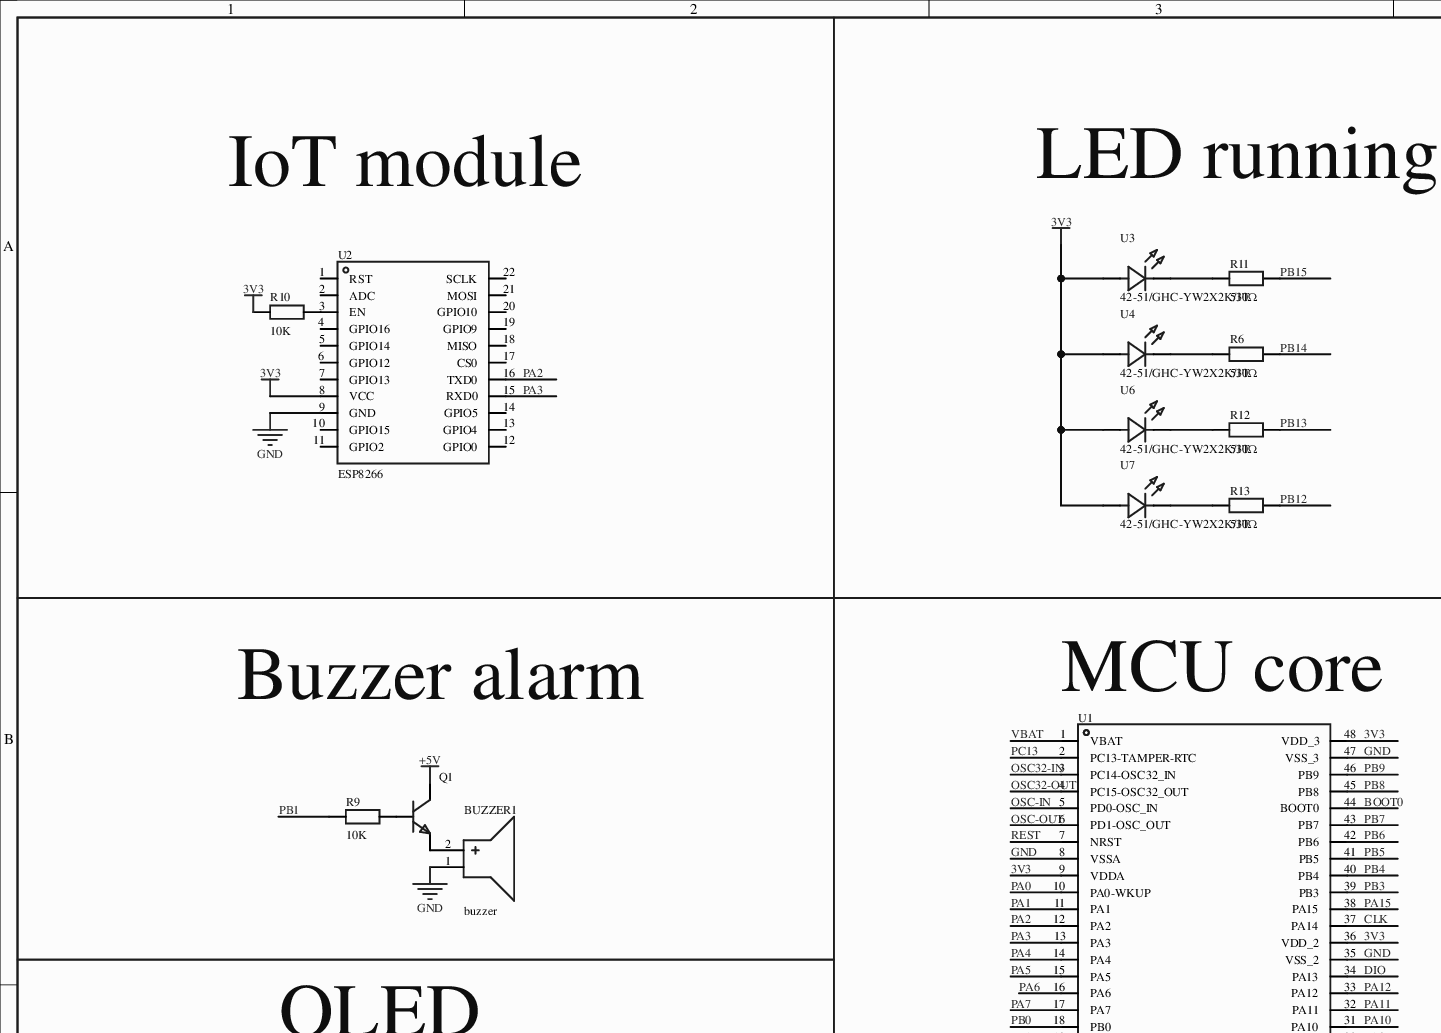
[diagram p0: MISC61952-3.schdoc, top left]
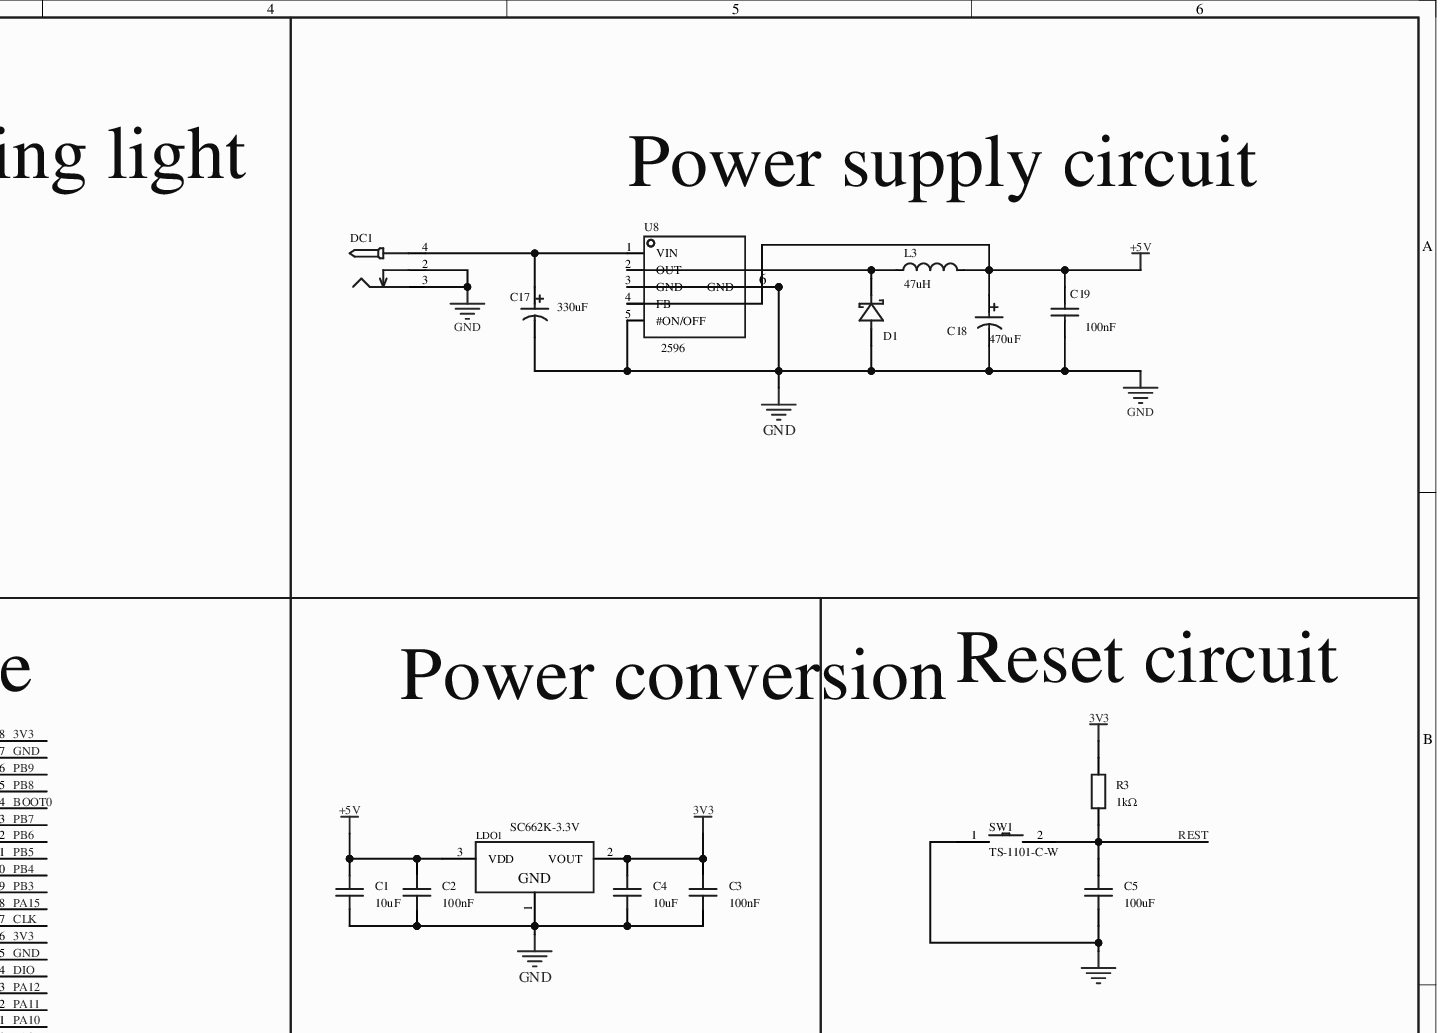
[diagram p1: MISC61952-3.schdoc, top right]
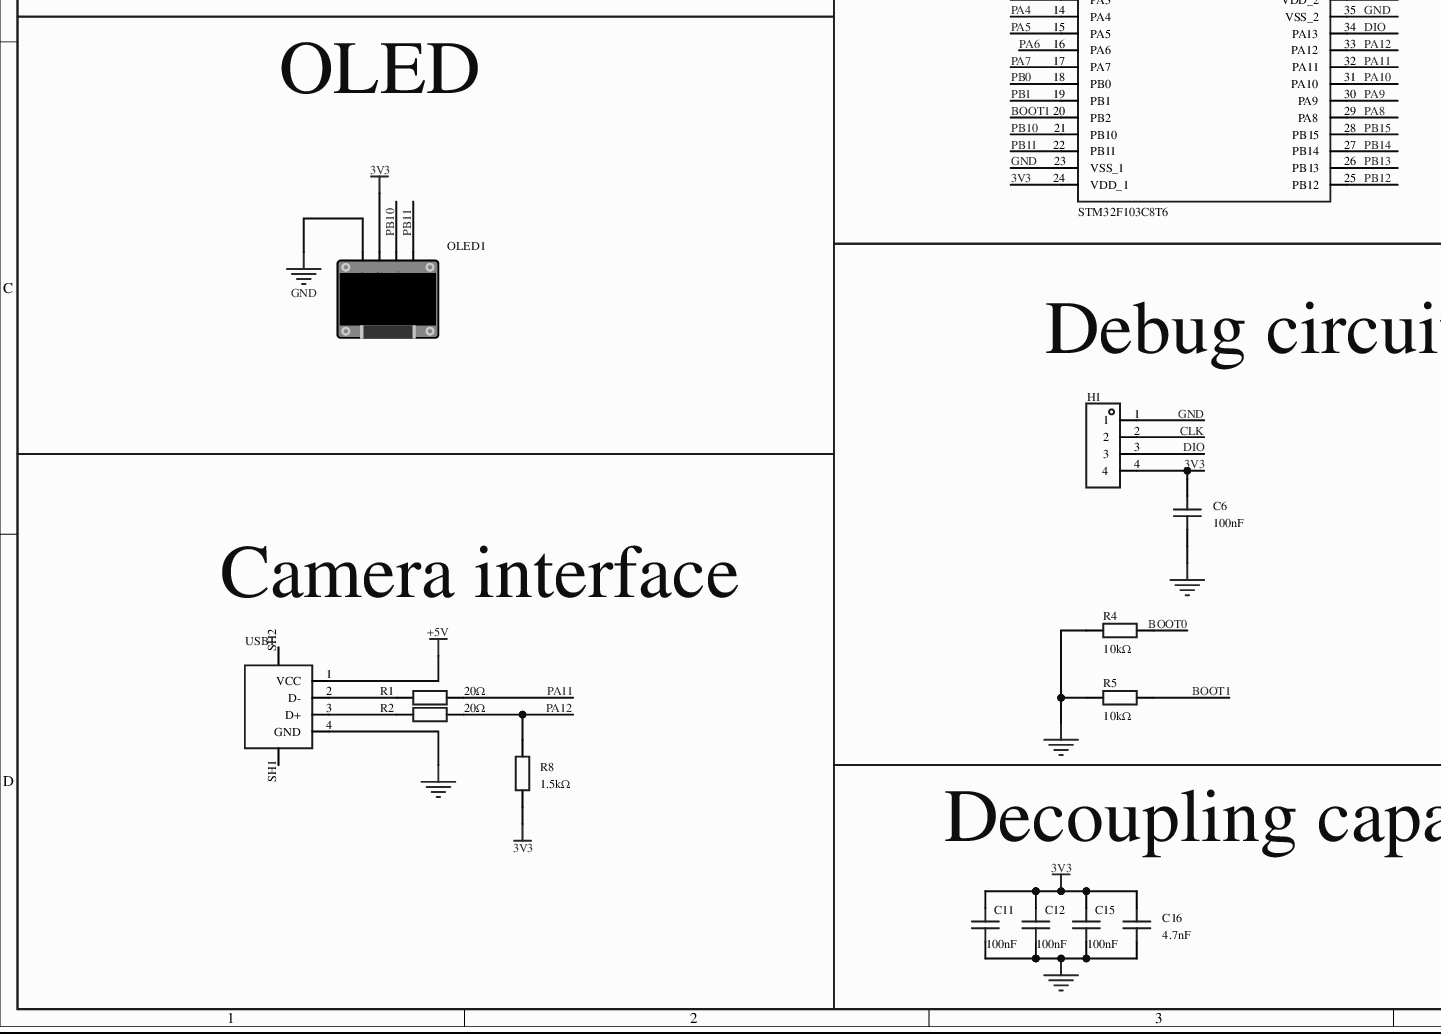
[diagram p2: MISC61952-3.schdoc, bottom left]
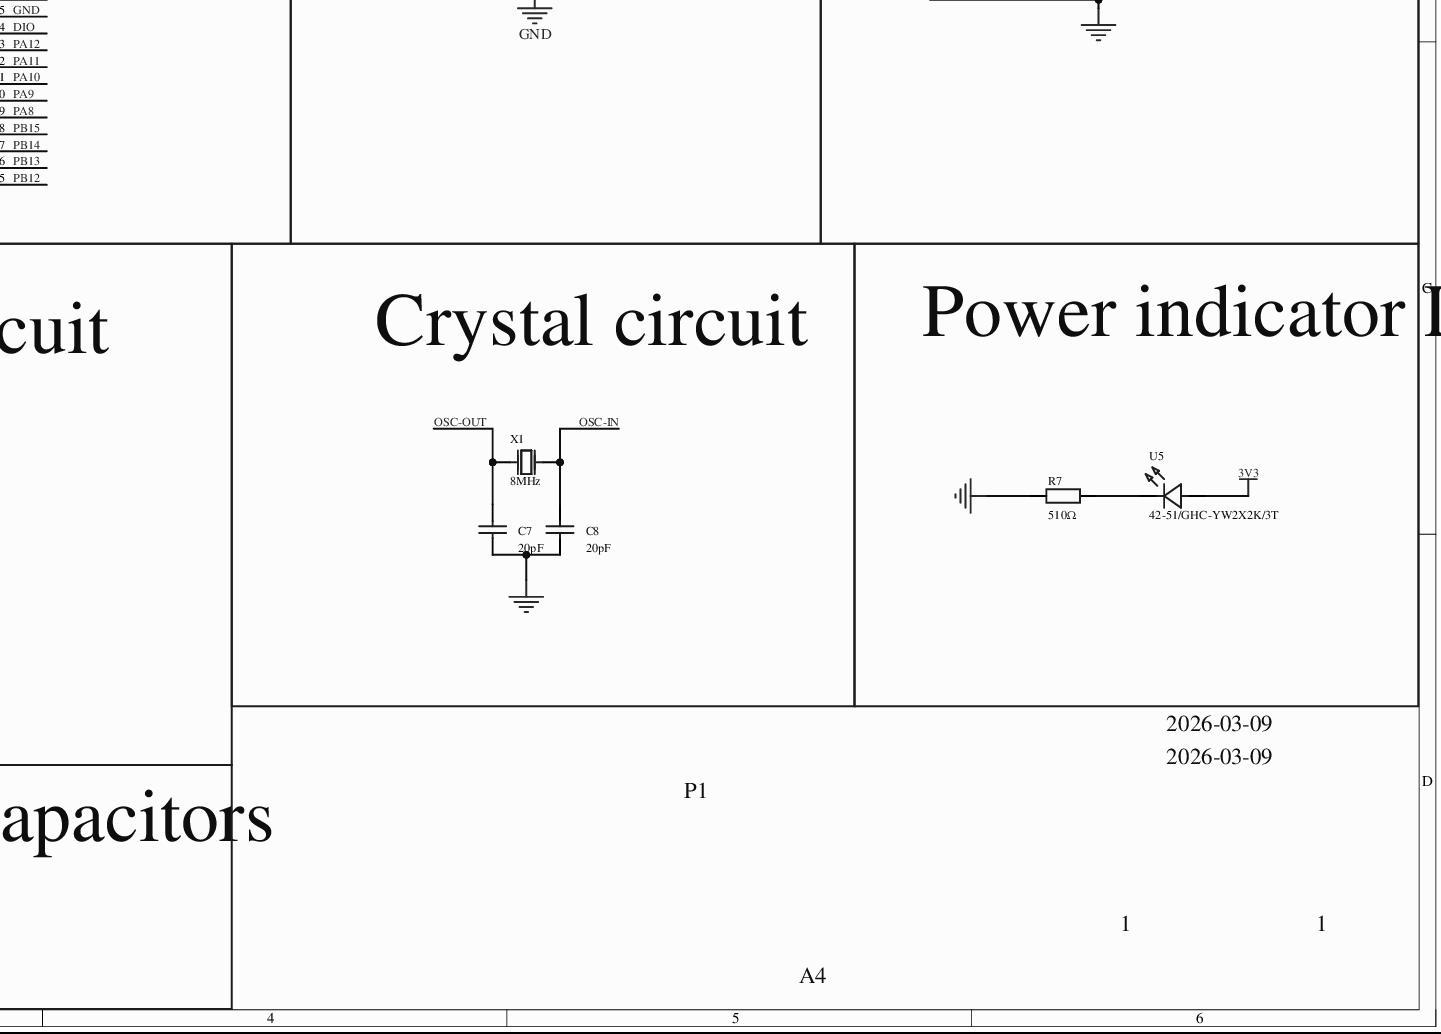
[diagram p3: MISC61952-3.schdoc, bottom right]
# Altium project MISC61952-2.PrjPcb
1 sheet, 47 parts. Net scope: global (net labels, ports and power ports of the same name join across sheets).
Board file: MISC61952.pcbdoc

## Sheet MISC61952-3.schdoc
size 420 x 297 mm; Version: V1.0; @Project Name: MISC61952; @Page Count: 1; @Update Date: 2026-03-09; @Create Date: 2026-03-09; @Schematic Name: MISC61952; @Page No: 1; @Board Name: MISC61952; @Create Time: 07:18:17; @Update Time: 19:34:13

### Parts
BUZZER1  buzzer  [BUZ-TH_BD12.0-P6.00-D0.9-RD]
C1  10uF  [C0603]
C2  100nF  [C0603]
C3  100nF  [C0603]
C4  10uF  [C0603]
C5  100uF  [C1206]
C6  100nF  [C0603]
C7  20pF  [C0603]
C8  20pF  [C0603]
C11  100nF  [C0603]
C12  100nF  [C0603]
C15  100nF  [C0603]
C16  4.7nF  [C0603]
C17  value 330uF  [CAP-SMD_BD8.0-L8.3-W8.3-RD]
C18  value 470uF  [CAP-SMD_BD8.0-L8.3-W8.3-RD]
C19  value 100nF  [C0805]
D1  (no value)  [SMA_L4.3-W2.6-LS5.2-RD]
DC1  (no value)  [DC-2.0]
H1  (no value)  [HDR-TH_4P-P2.54-V-M]
L3  value 47uH  [IND-SMD_L7.0-W6.6]
LDO1  SC662K-3.3V  [SOT-23-3_L2.9-W1.3-P1.90-LS2.4-BR]
OLED1  (no value)  [0.96OLED_4P]
Q1  (no value)  [S8050_SOT-23]
R1  20Ω  [R0603]
R2  20Ω  [R0603]
R3  1kΩ  [R0603]
R4  10kΩ  [R0603]
R5  10kΩ  [R0603]
R6  510Ω  [R0603]
R7  510Ω  [R0603]
R8  1.5kΩ  [R0603]
R9  10K  [R0603]
R10  10K  [R0603]
R11  510Ω  [R0603]
R12  510Ω  [R0603]
R13  510Ω  [R0603]
SW1  TS-1101-C-W  [SW-SMD_L6.0-W3.3-LS8.0]
U1  STM32F103C8T6  [LQFP-48_L7.0-W7.0-P0.50-LS9.0-BL]
U2  ESP8266  [WIFIM-SMD_ESP-12F-ESP8266MOD]
U3  42-51/GHC-YW2X2K/3T  [LED-SMD_L1.6-W0.8-FD_GREEN-1]
U4  42-51/GHC-YW2X2K/3T  [LED-SMD_L1.6-W0.8-FD_GREEN-1]
U5  42-51/GHC-YW2X2K/3T  [LED-SMD_L1.6-W0.8-FD_GREEN-1]
U6  42-51/GHC-YW2X2K/3T  [LED-SMD_L1.6-W0.8-FD_GREEN-1]
U7  42-51/GHC-YW2X2K/3T  [LED-SMD_L1.6-W0.8-FD_GREEN-1]
U8  LM2596S-5.0  [TO-263-5_L10.2-W8.9-P1.70-BR]  (value not drawn)
USB1  (no value)  [USB_ Type-A]
X1  8MHz  [OSC-TH_L10.0-W4.5-P5.00]

### Blocks framed on the sheet
IoT module: R10 U2
LED running light: R6 R11-R13 U3 U4 U6 U7
Power supply circuit: C17-C19 D1 DC1 L3 U8
Buzzer alarm: BUZZER1 Q1 R9
MCU core: U1
Power conversion: C1-C4 LDO1
Reset circuit: C5 R3 SW1
OLED: OLED1
Debug circuit: C6 H1 R4 R5
Crystal circuit: C7 C8 X1
Power indicator LED: R7 U5
Camera interface: R1 R2 R8 USB1
Decoupling capacitors: C11 C12 C15 C16

### Nets
3V3: C3.2 C4.2 C6.2 C11.2 C12.2 C15.2 C16.2 H1.4 LDO1.2(VOUT) OLED1.2(VCC) R3.2 R8.1 R10.1 U1.9(VDDA) U1.24(VDD_1) U1.36(VDD_2) U1.48(VDD_3) U2.8(VCC) U3.1(A) U4.1(A) U5.1(A) U6.1(A) U7.1(A)
+5V: C1.2 C2.2 C18.1 C19.1 L3.2 LDO1.3(VDD) Q1.3 U8.4(FB) USB1.1(VCC)
GND: BUZZER1.1(-) C1.1 C2.1 C3.1 C4.1 C5.1 C6.1 C7.1 C8.1 C11.1 C12.1 C15.1 C16.1 C17.2 C18.2 C19.2 D1.2(A) DC1.2 DC1.3 H1.1 LDO1.1(GND) OLED1.1(GND) R4.1 R5.1 R7.2 SW1.1 U1.8(VSSA) U1.23(VSS_1) U1.35(VSS_2) U1.47(VSS_3) U2.9(GND) U8.3(GND) U8.5(#ON/OFF) U8.6(GND) USB1.4(GND)
BOOT0: R4.2 U1.44(BOOT0)
BOOT1: R5.2 U1.20(PB2)
CLK: H1.2 U1.37(PA14)
DIO: H1.3 U1.34(PA13)
OSC32-IN: U1.3(PC14-OSC32_IN)
OSC32-OUT: U1.4(PC15-OSC32_OUT)
OSC-IN: C8.2 U1.5(PD0-OSC_IN) X1.1(OSC1)
OSC-OUT: C7.2 U1.6(PD1-OSC_OUT) X1.2(OSC2)
PA0: U1.10(PA0-WKUP)
PA1: U1.11(PA1)
PA2: U1.12(PA2) U2.16(TXD0)
PA3: U1.13(PA3) U2.15(RXD0)
PA4: U1.14(PA4)
PA5: U1.15(PA5)
PA6: U1.16(PA6)
PA7: U1.17(PA7)
PA8: U1.29(PA8)
PA9: U1.30(PA9)
PA10: U1.31(PA10)
PA11: R1.2 U1.32(PA11)
PA12: R2.2 R8.2 U1.33(PA12)
PA15: U1.38(PA15)
PB0: U1.18(PB0)
PB1: R9.1 U1.19(PB1)
PB3: U1.39(PB3)
PB4: U1.40(PB4)
PB5: U1.41(PB5)
PB6: U1.42(PB6)
PB7: U1.43(PB7)
PB8: U1.45(PB8)
PB9: U1.46(PB9)
PB10: OLED1.3(SCL) U1.21(PB10)
PB11: OLED1.4(SDA) U1.22(PB11)
PB12: R13.2 U1.25(PB12)
PB13: R12.2 U1.26(PB13)
PB14: R6.2 U1.27(PB14)
PB15: R11.2 U1.28(PB15)
PC13: U1.2(PC13-TAMPER-RTC)
REST: C5.2 R3.1 SW1.2 U1.7(NRST)
VBAT: U1.1(VBAT)
NetBUZZER1_2: BUZZER1.2(+) Q1.2
NetC17_1: C17.1 DC1.4 U8.1(VIN)
NetD1_1: D1.1(K) L3.1 U8.2(OUT)
NetQ1_1: Q1.1 R9.2
NetR1_1: R1.1 USB1.2(D-)
NetR2_1: R2.1 USB1.3(D+)
NetR6_1: R6.1 U4.2(C)
NetR7_1: R7.1 U5.2(C)
NetR10_2: R10.2 U2.3(EN)
NetR11_1: R11.1 U3.2(C)
NetR12_1: R12.1 U6.2(C)
NetR13_1: R13.1 U7.2(C)

Not connected (* = marked no-connect by the designer): U2 1(RST) 2(ADC) 4(GPIO16) 5(GPIO14) 6(GPIO12) 7(GPIO13) 10(GPIO15) 11(GPIO2) 12(GPIO0) 13(GPIO4) 14(GPIO5) 17(CS0) 18(MISO) 19(GPIO9) 20(GPIO10) 21(MOSI) 22(SCLK); USB1 SH1 SH2

### Notes on the sheet
- 2026-03-09
- P1
- A4
- 1

### Library data of the parts
BUZZER1 = buzzer: AddInBom: yes; ModelId: af17e4151ed84fc2a628230bf23763630819f05c4eef4c71ace90d822a990e87; ModelTransform: 472.44,472.176,0,270,0,0,0,0,-196.85; Symbol: BUZZER; Device: buzzer; LCSC Part Name: buzzer; SupplierPart: C9900014030; ManufacturerPart: buzzer; Supplier Footprint: buzzer; JLCPCB Part Class: Extended Part; Supplier: LCSC; ConvertToPcb: yes; FootprintName: BUZ-TH_BD12.0-P6.00-D0.9-RD; ModelName: BUZ-TH_BD12.0-P6.00-D0.9-RD
C1 C4 = CL10A106KP8NNNC: Capacitance: 10uF; tolerance: ±10%; rated voltage: 10V; dielectric (temperature coefficient): X5R;; Manufacturer: SAMSUNG(三星); AddInBom: yes; ModelId: ac125912035d415993ca9572d50418b1; ModelName: C0603_L1.6-W0.8-H0.8; ModelTransform: 62.992,31.496,0,0,0,0,0,0,0; Device: CL10A106KP8NNNC; Symbol: CL10A106KP8NNNC; LCSC Part Name: 10uF ±10% 10V; SupplierPart: C19702; ManufacturerPart: CL10A106KP8NNNC; Supplier Footprint: 0603; JLCPCB Part Class: Basic library; Datasheet: example.com/upload/public/pdf/source/20160103/1457707703378.pdf; Supplier: LCSC; ConvertToPcb: yes; FootprintName: C0603; Value: 10uF; Tolerance: ±10%; Voltage Rated: 10V; Temperature Coefficient: X5R
C2 C3 = CC0603KRX7R9BB104: Capacitance: 100nF; tolerance: ±10%; rated voltage: 50V; dielectric (temperature coefficient): X7R;; Manufacturer: YAGEO(国巨); AddInBom: yes; ModelId: ac125912035d415993ca9572d50418b1; ModelName: C0603_L1.6-W0.8-H0.8; ModelTransform: 62.992,31.496,0,0,0,0,0,0,0; Device: CC0603KRX7R9BB104; Symbol: CC0603KRX7R9BB104; LCSC Part Name: 100nF ±10% 50V; SupplierPart: C14663; ManufacturerPart: CC0603KRX7R9BB104; Supplier Footprint: 0603; JLCPCB Part Class: Basic library; Datasheet: example.com/upload/public/pdf/source/20180910/C282072_33301C7F631E79921B82A8DAC6BCC5B3.pdf; Supplier: LCSC; ConvertToPcb: yes; FootprintName: C0603; Value: 100nF; Tolerance: ±10%; Voltage Rated: 50V; Temperature Coefficient: X7R
C5 = HGC1206R5107M100NSPJ: Capacitance: 100uF; tolerance: ±20%; rated voltage: 10V; dielectric (temperature coefficient): X5R;; Manufacturer: Chinocera(华瓷); AddInBom: yes; ModelId: e4be705b945545a48e666415e3682bd8; ModelName: C1206_L3.2-W1.6-H1.3; ModelTransform: 125.984,62.992,0,0,0,0,0,0,0; Symbol: HGC1206R5107M100NSPJ; Device: HGC1206R5107M100NSPJ; LCSC Part Name: 100uF ±20% 10V; SupplierPart: C7432784; ManufacturerPart: HGC1206R5107M100NSPJ; Supplier Footprint: 1206; JLCPCB Part Class: Extended library; Datasheet: example.com/upload/public/pdf/source/20240320/FAC3FEC40A78BC5CCCE96C232A94D860.pdf; Supplier: LCSC; ConvertToPcb: yes; FootprintName: C1206; Value: 100uF; Tolerance: ±20%; Voltage Rated: 10V; Temperature Coefficient: X5R
C6 C11 C12 C15 = CGA0603X7R104K500JT: Capacitance: 100nF; tolerance: ±10%; rated voltage: 50V; dielectric (temperature coefficient): X7R;; Manufacturer: HRE(芯声); AddInBom: yes; ModelId: ac125912035d415993ca9572d50418b1; ModelName: C0603_L1.6-W0.8-H0.8; ModelTransform: 62.992,31.496,0,0,0,0,0,0,0; Symbol: CGA0603X7R104K500JT; Device: CGA0603X7R104K500JT; LCSC Part Name: 100nF ±10% 50V; SupplierPart: C6119867; ManufacturerPart: CGA0603X7R104K500JT; Supplier Footprint: 0603; JLCPCB Part Class: Extended library; Supplier: LCSC; ConvertToPcb: yes; FootprintName: C0603; Value: 100nF; Tolerance: ±10%; Voltage Rated: 50V; Temperature Coefficient: X7R
C7 C8 = CL10C200JB8NNNC: Capacitance: 20pF; tolerance: ±5%; rated voltage: 50V; dielectric (temperature coefficient): C0G;; Manufacturer: SAMSUNG(三星); AddInBom: yes; ModelId: ac125912035d415993ca9572d50418b1; ModelName: C0603_L1.6-W0.8-H0.8; ModelTransform: 62.992,31.496,0,0,0,0,0,0,0; Symbol: CL10C200JB8NNNC; Device: CL10C200JB8NNNC; LCSC Part Name: 20pF ±5% 50V; SupplierPart: C1648; ManufacturerPart: CL10C200JB8NNNC; Supplier Footprint: 0603; JLCPCB Part Class: Basic library; Datasheet: example.com/upload/public/pdf/source/20160218/1457707763339.pdf; Supplier: LCSC; ConvertToPcb: yes; FootprintName: C0603; Value: 20pF; Tolerance: ±5%; Voltage Rated: 50V; Temperature Coefficient: C0G
C16 = CGA0603X7R472K500JT: Capacitance: 4.7nF; tolerance: ±10%; rated voltage: 50V; dielectric (temperature coefficient): X7R;; Manufacturer: HRE(芯声); AddInBom: yes; ModelId: ac125912035d415993ca9572d50418b1; ModelName: C0603_L1.6-W0.8-H0.8; ModelTransform: 62.992,31.496,0,0,0,0,0,0,0; Symbol: CGA0603X7R472K500JT; Device: CGA0603X7R472K500JT; LCSC Part Name: 4.7nF ±10% 50V; SupplierPart: C7503499; ManufacturerPart: CGA0603X7R472K500JT; Supplier Footprint: 0603; JLCPCB Part Class: Extended library; Supplier: LCSC; ConvertToPcb: yes; FootprintName: C0603; Value: 4.7nF; Tolerance: ±10%; Voltage Rated: 50V; Temperature Coefficient: X7R
C17 C18 = CS1V221M-CRF10　: Capacitance: 220uF; tolerance: ±20%; rated voltage: 35V; can diameter: 8mm; can length: 10.5mm; ripple current: -; ESR: -; operating life: 2000hrs@105; operating temperature: -40~+105;; Manufacturer: ST(先科); Rated Voltage: 25V; 3D Model: b102f1362be24624a1b1334fec8dc7f4; 3D Model Transform: 354.33,326.81037,0,0,0,0,0,0,0; AddInBom: yes; Symbol: CS1V221M-CRF10; Device: CS1V221M-CRF10; Lifetime @ Temp: 2000hrs@105; Operating Temperature: -40~+105; Manufacturer Part: CS1V221M-CRF10; Supplier Footprint: SMD,8x10.5mm; JLCPCB Part Class: Extended Part; Datasheet: example.com/upload/public/pdf/source/20170325/1490427945143.pdf; Supplier: LCSC; Tolerance: ±20%; φD: 8mm; L: 10.5mm; Ripple Current: -; Equivalent Series Resistance(ESR): -; ConvertToPcb: yes; FootprintName: CAP-SMD_BD8.0-L8.3-W8.3-RD; ModelName: CAP-SMD_BD8.0-L8.3-W8.3-RD
  C17: Supplier Part: C97814
C19 = CL21B104KBCNNNC: Capacitance: 100nF; tolerance: ±10%; rated voltage: 50V; temperature coefficient: X7R;; Manufacturer: SAMSUNG(三星); 3D Model: 1ba041120af144c991958decab20d241; 3D Model Transform: 78.74,51.181,0,0,0,0,0,0.0005,0; AddInBom: yes; ModelName: C0805_L2.0-W1.3-H1.3; Symbol: CL21B104KBCNNNC; Device: CL21B104KBCNNNC; LCSC Part Name: 100nF ±10% 50V; Supplier Part: C1711; Manufacturer Part: CL21B104KBCNNNC; Supplier Footprint: 0805; JLCPCB Part Class: Extended Part; Datasheet: example.com/upload/public/pdf/source/20160103/1457707693305.pdf; Supplier: LCSC; Tolerance: ±10%; Voltage Rated: 50V; Temperature Coefficient: X7R; ConvertToPcb: yes; FootprintName: C0805
D1 = SS34_3: Manufacturer: TDD(台冠电子); Manufacturer Part: SS34; Symbol: SS34_C3032484; 3D Model: 7ed2c9d0a4a74bbdbba07ab4052caf5b; 3D Model Transform: 185.039,102.362,0,0,0,0,0,0,0; AddInBom: yes; Device: SS34_3; LCSC Part Name: SS34; Supplier Part: C3032484; Supplier Footprint: SMA; JLCPCB Part Class: Extended Part; Datasheet: example.com/upload/public/pdf/source/20220622/9D70D0693761B542BF6F533590093AA5.pdf; Supplier: LCSC; ConvertToPcb: yes; FootprintName: SMA_L4.3-W2.6-LS5.2-RD; ModelName: SMA_L4.3-W2.6-LS5.2-RD
DC1 = DC-005_2.0: Symbol: DC power jack; ConvertToPcb: yes; ModelId: f5f20b8a2308479b936ba3c2698865bb0819f05c4eef4c71ace90d822a990e87; ModelName: DC-IN-TH_DC-5520-1; ModelTransform: 372.05,551.18,582.68,90,0,0,137.8,0,-149.61; Device: DC-005_2.0; AddInBom: yes; Supplier Footprint: 插件; FootprintName: DC-2.0
H1 = HDR-M_2.54_1x4P: Symbol: PZ254V-11-04P; ConvertToPcb: yes; ModelId: 112f4d05e8d64e99ab9a333894bea4f90819f05c4eef4c71ace90d822a990e87; ModelName: HDR-TH_4P-P2.54-M-LI-1X4P; ModelTransform: 399.999,104.7242,0,0,0,0,0,0,-118.11; Device: HDR-M_2.54_1x4P; AddInBom: yes; SupplierPart: C492403; Supplier Footprint: 插件; FootprintName: HDR-TH_4P-P2.54-V-M
L3 = CMLO0630H330MTT: Inductance: 33uH; tolerance: ±20%; DC resistance (DCR): 270mΩ;; Manufacturer: Cybermax(思博科技); 3D Model: 6860c29aec394a38a0f014af7f722a42; 3D Model Transform: 275.6,259.8,0,0,0,0,0,0,0; AddInBom: yes; ModelName: IND-SMD_L7.0-W6.6-H3.0; Symbol: CMLO0630H330MTT; Device: CMLO0630H330MTT; LCSC Part Name: 33uH ±20% 270mΩ; Manufacturer Part: CMLO0630H330MTT; Supplier Footprint: SMD; JLCPCB Part Class: Extended Part; Datasheet: example.com/upload/public/pdf/source/20201124/C961478_55C23F293F63DC1D2CF3D7AB16D0E182.pdf; Supplier: LCSC; Tolerance: ±20%; DC Resistance (DCR): 270mΩ; ConvertToPcb: yes; FootprintName: IND-SMD_L7.0-W6.6
LDO1 = SC662K-3.3V: Output type: fixed; output polarity: positive; max input voltage: 6V; output voltage: 3.3V; output current: 250mA; power supply rejection ratio (PSRR): 50dB@(1kHz);; Manufacturer: FM(富满); AddInBom: yes; ModelId: c62791f0466c4ae2a892c056b845b0ca; ModelName: SOT-23-3P_L2.9-W1.3-H1.0-LS2.4-P0.95; ModelTransform: 98.425,114.173,0,180,0,0,0.0005,-0.0005,0; Number of Outputs: 1; Dropout Voltage: 38mV@(10mA); Symbol: SC662K-3.3V; Device: SC662K-3.3V; Supplier: LCSC; Manufacturer Part: SC662K-3.3V; Supplier Part: C83932; JLCPCB Part Class: Extended library; LCSC Part Name: 输入6V 输出3.3V 250mA 停产; Supplier Footprint: SOT-23; Datasheet: example.com/upload/public/pdf/source/20161024/1477288576049.pdf; ConvertToPcb: yes; FootprintName: SOT-23-3_L2.9-W1.3-P1.90-LS2.4-BR; Output Type: Fixed; Output Polarity: Positive; Maximum Input Voltage: 6V; Output Voltage: 3.3V; Output Current: 250mA; Power Supply Rejection Ratio (PSRR): 50dB@(1kHz)
OLED1 = 0.96OLED模块_4P: Symbol: 0.96OLED module_4P; ConvertToPcb: yes; ModelId: 79c000fdb68d45a296c2e9bedf4f90550819f05c4eef4c71ace90d822a990e87; ModelTransform: 1393.69792,1318.895,0,0,0,0,0,-560.079,-137.795; Device: 0.96OLED module_4P; AddInBom: yes; FootprintName: 0.96OLED_4P; Supplier Footprint: 插件; ModelName: 0.96OLED_4P
Q1 = S8050_SOT_NPN: Symbol: NPN; ConvertToPcb: yes; ModelId: c62791f0466c4ae2a892c056b845b0ca0819f05c4eef4c71ace90d822a990e87; ModelName: SOT-23-3P_L2.9-W1.3-H1.0-LS2.4-P0.95; ModelTransform: 98.6,114.12,41.29,180,0,0,0,0,-3; Device: S8050_SOT_NPN; AddInBom: yes; Supplier Footprint: SOT-23; FootprintName: S8050_SOT-23
R1 R2 = 0603WAF200JT5E: Resistor type: thick film resistor; resistance: 20Ω; tolerance: ±1%; power: 100mW; max working voltage: 75V; temperature coefficient: ±100ppm/℃;; Manufacturer: UNI-ROYAL(厚声); AddInBom: yes; ModelId: fc143cca1e79419f9cd78b61e9279f08; ModelTransform: 31.8897,63.7794,0,90,0,0,0,0,0; Symbol: 0603WAF200JT5E; Device: 0603WAF200JT5E; LCSC Part Name: 20Ω ±1% 100mW 厚膜电阻; SupplierPart: C22950; ManufacturerPart: 0603WAF200JT5E; Supplier Footprint: 0603; JLCPCB Part Class: Basic library; Datasheet: example.com/upload/public/pdf/source/20200306/C422600_1E6D84923E4A46A82E41ADD87F860B5C.pdf; Supplier: LCSC; ConvertToPcb: yes; FootprintName: R0603; ModelName: R0603; Type: Thick film resistor; Value: 20Ω; Tolerance: ±1%; Power(Watts): 100mW; Overload Voltage (Max): 75V; Temperature Coefficient: ±100ppm/℃; Operating Temperature Range: -55℃~+155℃
R3 = RC0603FR-071KL: Resistor type: thick film resistor; resistance: 1kΩ; tolerance: ±1%; power: 100mW; max working voltage: 75V; temperature coefficient: ±100ppm/℃;; Manufacturer: YAGEO(国巨); AddInBom: yes; ModelId: fc143cca1e79419f9cd78b61e9279f08; ModelTransform: 31.8897,63.7794,0,90,0,0,0,0,0; Symbol: RC0603FR-071KL; Device: RC0603FR-071KL; LCSC Part Name: 厚膜电阻 1kΩ ±1% 100mW; SupplierPart: C22548; ManufacturerPart: RC0603FR-071KL; Supplier Footprint: 0603; JLCPCB Part Class: Extended library; Datasheet: example.com/upload/public/pdf/source/20180316/70C0E2BDAE7FCC62C531A5A58D202EE1.pdf; Supplier: LCSC; ConvertToPcb: yes; FootprintName: R0603; ModelName: R0603; Type: Thick film resistor; Value: 1kΩ; Tolerance: ±1%; Power(Watts): 100mW; Overload Voltage (Max): 75V; Temperature Coefficient: ±100ppm/℃; Operating Temperature Range: -55℃~+155℃
R4 R5 = 0603WAF1002T5E: Resistor type: thick film resistor; resistance: 10kΩ; tolerance: ±1%; power: 100mW; max working voltage: 75V; temperature coefficient: ±100ppm/℃;; Manufacturer: UNI-ROYAL(厚声); AddInBom: yes; ModelId: fc143cca1e79419f9cd78b61e9279f08; ModelTransform: 31.8897,63.7794,0,90,0,0,0,0,0; Symbol: 0603WAF1002T5E; Device: 0603WAF1002T5E; LCSC Part Name: 厚膜电阻 10kΩ ±1% 100mW; SupplierPart: C25804; ManufacturerPart: 0603WAF1002T5E; Supplier Footprint: 0603; JLCPCB Part Class: Basic library; Datasheet: example.com/upload/public/pdf/source/20200306/C422600_1E6D84923E4A46A82E41ADD87F860B5C.pdf; Supplier: LCSC; ConvertToPcb: yes; FootprintName: R0603; ModelName: R0603; Type: Thick film resistor; Value: 10kΩ; Tolerance: ±1%; Power(Watts): 100mW; Overload Voltage (Max): 75V; Temperature Coefficient: ±100ppm/℃; Operating Temperature Range: -55℃~+155℃
R6 R11-R13 = 0603WAF5100T5E: Resistor type: thick film resistor; resistance: 510Ω; tolerance: ±1%; power: 100mW; max working voltage: 75V; temperature coefficient: ±100ppm/℃;; Manufacturer: UNI-ROYAL(厚声); 3D Model: fc143cca1e79419f9cd78b61e9279f08; 3D Model Transform: 31.8897,63.7794,0,90,0,0,0,0,0; AddInBom: yes; Symbol: 0603WAF5100T5E; Device: 0603WAF5100T5E; LCSC Part Name: 510Ω ±1% 100mW 厚膜电阻; Supplier Part: C23193; Manufacturer Part: 0603WAF5100T5E; Supplier Footprint: 0603; JLCPCB Part Class: Basic library; Datasheet: example.com/upload/public/pdf/source/20200306/C422600_1E6D84923E4A46A82E41ADD87F860B5C.pdf; Supplier: LCSC; Type: Thick film resistor; Value: 510Ω; Tolerance: ±1%; Power(Watts): 100mW; Overload Voltage (Max): 75V; Temperature Coefficient: ±100ppm/℃; Operating Temperature Range: -55℃~+155℃; ConvertToPcb: yes; FootprintName: R0603; ModelName: R0603
R7 = 0603WAF5100T5E: Resistor type: thick film resistor; resistance: 510Ω; tolerance: ±1%; power: 100mW; max working voltage: 75V; temperature coefficient: ±100ppm/℃;; Manufacturer: UNI-ROYAL(厚声); AddInBom: yes; ModelId: fc143cca1e79419f9cd78b61e9279f08; ModelTransform: 31.8897,63.7794,0,90,0,0,0,0,0; Symbol: 0603WAF5100T5E; Device: 0603WAF5100T5E; LCSC Part Name: 510Ω ±1% 100mW 厚膜电阻; SupplierPart: C23193; ManufacturerPart: 0603WAF5100T5E; Supplier Footprint: 0603; JLCPCB Part Class: Basic library; Datasheet: example.com/upload/public/pdf/source/20200306/C422600_1E6D84923E4A46A82E41ADD87F860B5C.pdf; Supplier: LCSC; ConvertToPcb: yes; FootprintName: R0603; ModelName: R0603; Type: Thick film resistor; Value: 510Ω; Tolerance: ±1%; Power(Watts): 100mW; Overload Voltage (Max): 75V; Temperature Coefficient: ±100ppm/℃; Operating Temperature Range: -55℃~+155℃
R8 = 0603WAF1501T5E: Resistor type: thick film resistor; resistance: 1.5kΩ; tolerance: ±1%; power: 100mW; max working voltage: 75V; temperature coefficient: ±100ppm/℃;; Manufacturer: UNI-ROYAL(厚声); AddInBom: yes; ModelId: fc143cca1e79419f9cd78b61e9279f08; ModelTransform: 31.8897,63.7794,0,90,0,0,0,0,0; Symbol: 0603WAF1501T5E; Device: 0603WAF1501T5E; LCSC Part Name: 1.5kΩ ±1% 100mW 厚膜电阻; SupplierPart: C22843; ManufacturerPart: 0603WAF1501T5E; Supplier Footprint: 0603; JLCPCB Part Class: Basic library; Datasheet: example.com/upload/public/pdf/source/20200306/C422600_1E6D84923E4A46A82E41ADD87F860B5C.pdf; Supplier: LCSC; ConvertToPcb: yes; FootprintName: R0603; ModelName: R0603; Type: Thick film resistor; Value: 1.5kΩ; Tolerance: ±1%; Power(Watts): 100mW; Overload Voltage (Max): 75V; Temperature Coefficient: ±100ppm/℃; Operating Temperature Range: -55℃~+155℃
R9 R10 = Res_0603: Symbol: Resistor; ConvertToPcb: yes; ModelId: fc143cca1e79419f9cd78b61e9279f080819f05c4eef4c71ace90d822a990e87; ModelTransform: 31.8897,63.7794,0,90,0,0,0,0,0; Device: Res_0603; AddInBom: yes; Supplier Footprint: 0603; FootprintName: R0603; ModelName: R0603; Value: 10K
SW1 = TS-1101-C-W: Circuit structure: SPST; button shape: rectangular button; actuation force: 260gf; mounting: upright SMT; switch length: 6mm; switch width: 3.6mm; switch height: 2.5mm; with bracket: no; contact current: 50mA; rated voltage (AC): -; rated voltage (DC): 12V; rated power: -; insulation resistance: -; with lamp: no; mechanical life: 5 ten-thousand cycles;; Manufacturer: XKB Connectivity(中国星坤); AddInBom: yes; ModelId: b2f4ea9f0afc4b0786d53dba66ceb9e4; ModelName: SW-SMD_L6.0-W3.3-H5-LS8.0; ModelTransform: 314.96,129.921,0,0,0,0,0,0,0; Actuator/Cap Color: White with light green tint; Symbol: TS-1101-C-W; Device: TS-1101-C-W; LCSC Part Name: 6*3.6*2.5mm 立贴 轻触开关; SupplierPart: C318938; ManufacturerPart: TS-1101-C-W; Supplier Footprint: SMD; JLCPCB Part Class: Extended library; Datasheet: example.com/upload/public/pdf/source/20200227/C318938_C2E53B1EEDE37D980A33616AC086DE53.pdf; Supplier: LCSC; ConvertToPcb: yes; FootprintName: SW-SMD_L6.0-W3.3-LS8.0; Circuit: SPST; Actuator Style: Rectangular button; Operating Force: 260gf; Mounting Style: Upright SMT; Switch Length: 6mm; Switch Width: 3.6mm; Switch Height: 2.5mm; Strike Gundam: No; Contact Current: 50mA; Voltage Rating (AC): -; Voltage Rating (DC): 12V; Power Rating: -; Insulation Resistance: -; With Lamp: No; IP Rating: -; Pin Style: -; Mechanical Life: 5 ten-thousand cycles; Operating Temperature: -30℃~+85℃
U1 = STM32F103C8T6: CPU core: ARM-M3; program memory capacity: 64KB; RAM total capacity: 20KB; GPIO port count: 37; operating voltage range: 2V~3.6V; max CPU frequency: 72MHz; program memory type: FLASH;; Manufacturer: ST(意法半导体); AddInBom: yes; ModelId: 093be70396ff421eb2cdb946d5311efc; ModelName: LQFP-48_L7.0-W7.0-H1.4-LS9.0-P0.50; ModelTransform: 354.331,354.331,0,0,0,0,0,0,0; GPIO Ports Number: 37; ADC (Bit): 12bit; Peripheral/Function: Watchdog; DMA; Watchdog; Temperature sensor; Symbol: STM32F103C8T6; Device: STM32F103C8T6; LCSC Part Name: 主流增强型ARM Cortex-M3 MCU，具有64 KB Flash、72 MHz CPU、电机控制、USB和CAN; SupplierPart: C8734; ManufacturerPart: STM32F103C8T6; Supplier Footprint: LQFP-48(7x7); JLCPCB Part Class: Extended library; Datasheet: example.com/upload/public/pdf/source/20220812/8363ACEC51AD55ECEB84799464F7CB85.pdf; Supplier: LCSC; ConvertToPcb: yes; FootprintName: LQFP-48_L7.0-W7.0-P0.50-LS9.0-BL; CPU Core: ARM-M3; Program Storage Size: 64KB; RAM Size: 20KB; Operating Voltage Range: 2V~3.6V; CPU Maximum Speed: 72MHz; Program Memory Type: FLASH; Operating Temperature Range: -40℃~+85℃; DAC (Bit): -; PWM (Bit): -; Universal Serial Bus: Yes; Internal Comparator: -; communication protocol: -; Watchdog: Yes; Real-Time Clock: -; Infrared Data Association: Yes; Low-Voltage Detect: Yes; CCP Capture/Compare: -; Secure Digital Input and Output: -; Direct Memory Access: Yes; Internal Oscillator: Yes
U2 = ESP8266: AddInBom: yes; ModelId: c53b8c57aa74447bb5071c1a48f7c2190819f05c4eef4c71ace90d822a990e87; ModelName: WIFIM-SMD_WIFI-L24.0-W16.0-H3.1; ModelTransform: 630.707,945.274,0,90,0,0,-162.403,0,0; Symbol: ESP8266; Device: ESP8266; LCSC Part Name: ESP8266; SupplierPart: C9900003049; ManufacturerPart: ESP8266; Supplier Footprint: WIFIM-SMD; JLCPCB Part Class: Extended Part; Supplier: LCSC; ConvertToPcb: yes; FootprintName: WIFIM-SMD_ESP-12F-ESP8266MOD
U3 U4 U6 U7 = 42-51/GHC-YW2X2K/3T: Emitted color: emerald green; forward current: -; dominant wavelength: 520nm~535nm; luminous intensity: 2850mcd;; Manufacturer: EVERLIGHT(亿光); 3D Model: feee2acead2344579596fed70e7e7f0f; 3D Model Transform: 63.7794,31.89954,0,0,0,0,0,0,0; AddInBom: yes; Symbol: 42-51/GHC-YW2X2K/3T; Device: 42-51/GHC-YW2X2K/3T; LCSC Part Name: 正发光贴片灯 颜色正绿色 发光二极管; Supplier Part: C5136797; Manufacturer Part: 42-51/GHC-YW2X2K/3T; Supplier Footprint: 0603; JLCPCB Part Class: Extended library; Datasheet: example.com/upload/public/pdf/source/20220916/FBE88CF67A3FC292A254CF6ACE30EBDE.pdf; Supplier: LCSC; Emitted Color: Emerald green; Forward Current: -; Dominant Wavelength: 520nm~535nm; Luminous Intensity: 2850mcd; ConvertToPcb: yes; FootprintName: LED-SMD_L1.6-W0.8-FD_GREEN-1; ModelName: LED-SMD_L1.6-W0.8-FD_GREEN-1
U5 = 42-51/GHC-YW2X2K/3T: Emitted color: emerald green; forward current: -; dominant wavelength: 520nm~535nm; luminous intensity: 2850mcd;; Manufacturer: EVERLIGHT(亿光); AddInBom: yes; ModelId: feee2acead2344579596fed70e7e7f0f; ModelTransform: 63.7794,31.89954,0,0,0,0,0,0,0; Symbol: 42-51/GHC-YW2X2K/3T; Device: 42-51/GHC-YW2X2K/3T; LCSC Part Name: 正发光贴片灯 颜色正绿色 发光二极管; SupplierPart: C5136797; ManufacturerPart: 42-51/GHC-YW2X2K/3T; Supplier Footprint: 0603; JLCPCB Part Class: Extended library; Datasheet: example.com/upload/public/pdf/source/20220916/FBE88CF67A3FC292A254CF6ACE30EBDE.pdf; Supplier: LCSC; ConvertToPcb: yes; FootprintName: LED-SMD_L1.6-W0.8-FD_GREEN-1; ModelName: LED-SMD_L1.6-W0.8-FD_GREEN-1; Emitted Color: Emerald green; Forward Current: -; Dominant Wavelength: 520nm~535nm; Luminous Intensity: 2850mcd
U8 = LM2596S-5.0_C347421: Function type: step-down; output type: fixed; input voltage: 40V; output voltage: 5V; max output current: 3A;; Manufacturer: UMW(广东友台半导体); Symbol: LM2596-TO263; Add into BOM: yes; 3D Model: 4e421a816a7f4d57b8710832ddea550a; 3D Model Transform: 401.574,560.17797,0,90,0,0,-45.276,0,0; Synchronous Rectification: No; Number of Outputs: 1; Switching Frequency: 150kHz; ModelName: TO-263-5-5P_L10.2-W8.7-H4.5-LS14.4-P1.70; Device: LM2596S-5.0_C347421; Convert to PCB: yes; LCSC Part Name: 降压型 输入40V 输出5V 3A; Supplier Part: C347421; Manufacturer Part: LM2596S-5.0; Supplier Footprint: TO-263-5; JLCPCB Part Class: Extended Part; Datasheet: example.com/upload/public/pdf/source/20211011/C7416AEF3194BD283261B8F2553C4145.pdf; Supplier: LCSC; Function: Step-down; Output Type: Fixed; Topology: Step-down; Input Voltage: 40V; Output Voltage: 5V; Output Current (Max): 3A; Operating Temperature: -40℃~+125℃@(TA); FootprintName: TO-263-5_L10.2-W8.9-P1.70-BR
USB1 = USB_ Type-A: AddInBom: yes; ModelId: 0a0bfc60af8549fa93b7465d8aaf02b10819f05c4eef4c71ace90d822a990e87; ModelName: USB-A-TH__USB-AF-90; ModelTransform: 612.05,551.18,446.85,0,0,0,0,-15.75,-157.48; Symbol: USB_Type-A; Device: USB_ Type-A; ConvertToPcb: yes; FootprintName: USB_ Type-A; Supplier Footprint: 插件
X1 = X49SD8MSD2SC: Crystal type: through-hole crystal; frequency: 8MHz; room-temperature frequency deviation: ±20ppm; load capacitance: 20pF; frequency stability (full temperature): ±30ppm;; Manufacturer: YXC(扬兴晶振); AddInBom: yes; ModelId: a8e34f6c394c4d60ace7720f62d1ccdf; ModelName: HC-49US_L11.0-W4.5-H3.5-P4.88; ModelTransform: 432.46488,177.165,0,90,0,0,0,0,-137.795; Symbol: X49SD8MSD2SC; Device: X49SD8MSD2SC; LCSC Part Name: 8MHz ±20ppm 20pF; SupplierPart: C21263; ManufacturerPart: X49SD8MSD2SC; Supplier Footprint: HC-49S; JLCPCB Part Class: Extended library; Datasheet: example.com/upload/public/pdf/source/20240329/977D7F2434F98B2BE33270BB9FF3D86D.pdf; Supplier: LCSC; ConvertToPcb: yes; FootprintName: OSC-TH_L10.0-W4.5-P5.00; Crystal Type: Through-hole crystal; Value: 8MHz; Normal temperature Frequency Tolerance: ±20ppm; External load capacitor: 20pF; Frequency Stability(Full temperature range): ±30ppm; Operating Temperature: -20℃~+70℃